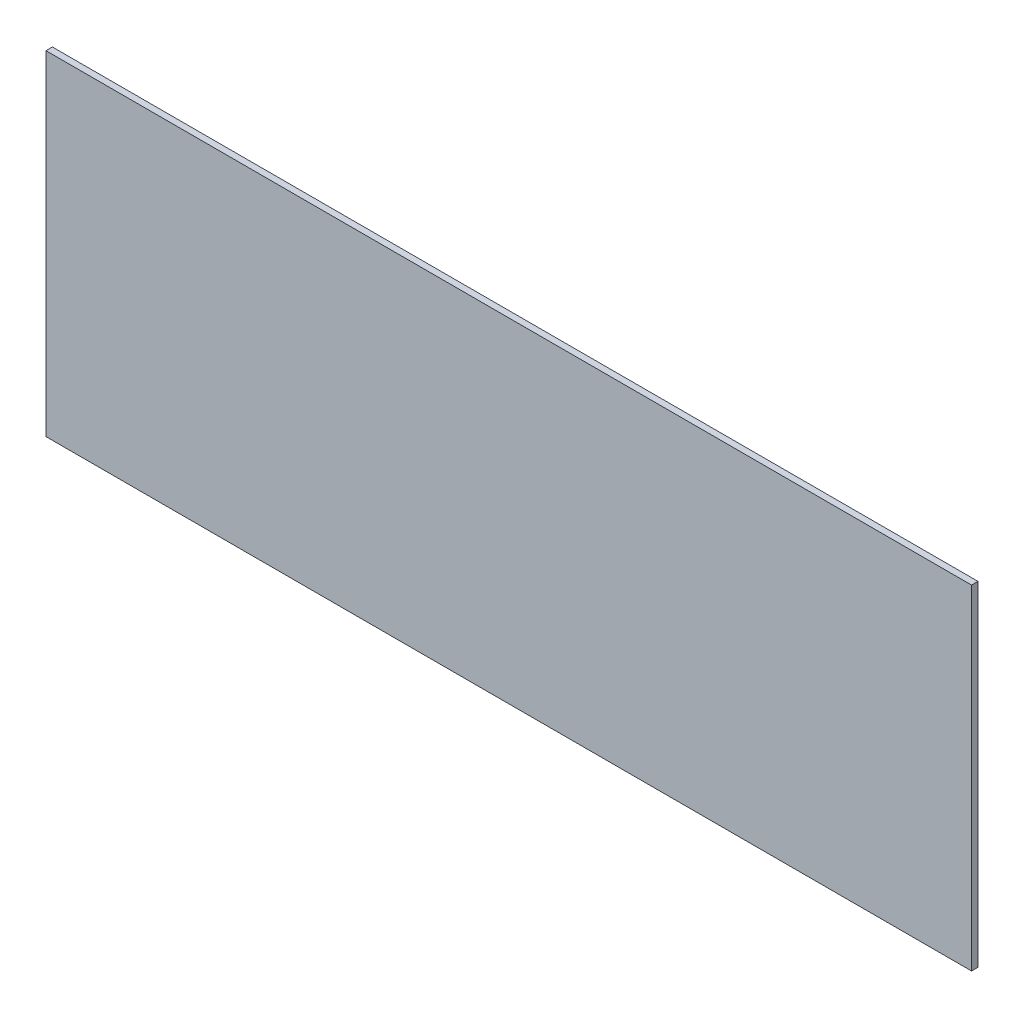
SolidWorks part; units mm, degrees
ref_plane "前视基准面" through (0, 0, 0) normal (0, 0, 1) x (1, 0, 0)
ref_plane "上视基准面" through (0, 0, 0) normal (0, 1, 0) x (1, 0, 0)
ref_plane "右视基准面" through (0, 0, 0) normal (1, 0, 0) x (0, 0, -1)
other "Configuration Table"
sketch "草图1" plane through (0, 0, 0) normal (0, 0, 1) x (1, 0, 0)
  line L1 (-360, -130) -> (360, -130)
  line L2 (-360, -130) -> (-360, 130)
  line L3 (-360, 130) -> (360, 130)
  line L4 (360, -130) -> (360, 130)
  line L5 (-360, -130) -> (360, 130) construction
  line L6 (-360, 130) -> (360, -130) construction
  point P0 (0, 0)
  dimension "D1" = 260
  dimension "D2" = 720
extrude "凸台-拉伸1" add sketch "草图1" along normal blind 5
